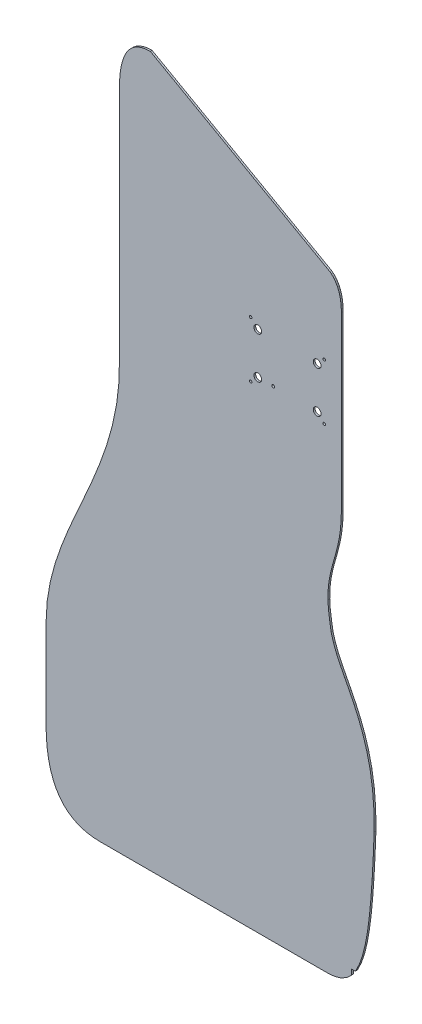
SolidWorks part; units mm, degrees
ref_plane "前视基准面" through (0, 0, 0) normal (0, 0, 1) x (1, 0, 0)
ref_plane "上视基准面" through (0, 0, 0) normal (0, 1, 0) x (1, 0, 0)
ref_plane "右视基准面" through (0, 0, 0) normal (1, 0, 0) x (0, 0, -1)
other "Configuration Table"
sketch "草图1" plane through (0, 0, 0) normal (0, 0, 1) x (1, 0, 0)
  line L0 (103, 235) -> (-24.8333, 235)
  line L1 (-24.8333, 235) -> (-152.6667, 235)
  line L2 (-152.6667, 235) -> (-280.5, 235)
  line L3 (-280.5, 235) -> (-293.0357, 235.6378)
  line L4 (-293.0357, 235.6378) -> (-304.6429, 237.551)
  line L5 (-304.6429, 237.551) -> (-315.3214, 240.7398)
  line L6 (-315.3214, 240.7398) -> (-325.0714, 245.2041)
  line L7 (-325.0714, 245.2041) -> (-333.8929, 250.9439)
  line L8 (-333.8929, 250.9439) -> (-341.7857, 257.9592)
  line L9 (-341.7857, 257.9592) -> (-348.75, 266.25)
  line L10 (-348.75, 266.25) -> (-354.7857, 275.8163)
  line L11 (-354.7857, 275.8163) -> (-359.8929, 286.6582)
  line L12 (-359.8929, 286.6582) -> (-364.0714, 298.7755)
  line L13 (-364.0714, 298.7755) -> (-367.3214, 312.1684)
  line L14 (-367.3214, 312.1684) -> (-369.6429, 326.8367)
  line L15 (-369.6429, 326.8367) -> (-371.0357, 342.7806)
  line L16 (-371.0357, 342.7806) -> (-371.5, 360)
  line L17 (-371.5, 360) -> (-371.5, 410)
  line L18 (-371.5, 410) -> (-371.5, 460)
  line L19 (-371.5, 460) -> (-371.5, 510)
  line L20 (-371.5, 510) -> (-369.6073, 541.7165)
  line L21 (-369.6073, 541.7165) -> (-364.3178, 572.7114)
  line L22 (-364.3178, 572.7114) -> (-356.2141, 603.1815)
  line L23 (-356.2141, 603.1815) -> (-345.879, 633.3236)
  line L24 (-345.879, 633.3236) -> (-333.8952, 663.3345)
  line L25 (-333.8952, 663.3345) -> (-320.8455, 693.4111)
  line L26 (-320.8455, 693.4111) -> (-307.3125, 723.75)
  line L27 (-307.3125, 723.75) -> (-293.879, 754.5481)
  line L28 (-293.879, 754.5481) -> (-281.1277, 786.0022)
  line L29 (-281.1277, 786.0022) -> (-269.6414, 818.309)
  line L30 (-269.6414, 818.309) -> (-260.0027, 851.6655)
  line L31 (-260.0027, 851.6655) -> (-252.7945, 886.2682)
  line L32 (-252.7945, 886.2682) -> (-248.5993, 922.3141)
  line L33 (-248.5993, 922.3141) -> (-248, 960)
  line L34 (-248, 960) -> (-248, 1090)
  line L35 (-248, 1090) -> (-248, 1220)
  line L36 (-248, 1220) -> (-248, 1350)
  line L37 (-248, 1350) -> (-247.7347, 1361.0204)
  line L38 (-247.7347, 1361.0204) -> (-246.9388, 1371.2245)
  line L39 (-246.9388, 1371.2245) -> (-245.6122, 1380.6122)
  line L40 (-245.6122, 1380.6122) -> (-243.7551, 1389.1837)
  line L41 (-243.7551, 1389.1837) -> (-241.3673, 1396.9388)
  line L42 (-241.3673, 1396.9388) -> (-238.449, 1403.8776)
  line L43 (-238.449, 1403.8776) -> (-235, 1410)
  line L44 (-235, 1410) -> (-231.0204, 1415.3061)
  line L45 (-231.0204, 1415.3061) -> (-226.5102, 1419.7959)
  line L46 (-226.5102, 1419.7959) -> (-221.4694, 1423.4694)
  line L47 (-221.4694, 1423.4694) -> (-215.898, 1426.3265)
  line L48 (-215.898, 1426.3265) -> (-209.7959, 1428.3673)
  line L49 (-209.7959, 1428.3673) -> (-203.1633, 1429.5918)
  line L50 (-203.1633, 1429.5918) -> (-196, 1430)
  line L51 (-196, 1430) -> (-95.25, 1373.3333)
  line L52 (-95.25, 1373.3333) -> (5.5, 1316.6667)
  line L53 (5.5, 1316.6667) -> (106.25, 1260)
  line L54 (106.25, 1260) -> (108.9362, 1257.8878)
  line L55 (108.9362, 1257.8878) -> (111.4235, 1255.551)
  line L56 (111.4235, 1255.551) -> (113.7117, 1252.9898)
  line L57 (113.7117, 1252.9898) -> (115.801, 1250.2041)
  line L58 (115.801, 1250.2041) -> (117.6913, 1247.1939)
  line L59 (117.6913, 1247.1939) -> (119.3827, 1243.9592)
  line L60 (119.3827, 1243.9592) -> (120.875, 1240.5)
  line L61 (120.875, 1240.5) -> (122.1684, 1236.8163)
  line L62 (122.1684, 1236.8163) -> (123.2628, 1232.9082)
  line L63 (123.2628, 1232.9082) -> (124.1582, 1228.7755)
  line L64 (124.1582, 1228.7755) -> (124.8546, 1224.4184)
  line L65 (124.8546, 1224.4184) -> (125.352, 1219.8367)
  line L66 (125.352, 1219.8367) -> (125.6505, 1215.0306)
  line L67 (125.6505, 1215.0306) -> (125.75, 1210)
  line L68 (125.75, 1210) -> (125.75, 1113.3333)
  line L69 (125.75, 1113.3333) -> (125.75, 1016.6667)
  line L70 (125.75, 1016.6667) -> (125.75, 920)
  line L71 (125.75, 920) -> (125.281, 904.7303)
  line L72 (125.281, 904.7303) -> (123.9876, 890.9038)
  line L73 (123.9876, 890.9038) -> (122.0405, 878.2799)
  line L74 (122.0405, 878.2799) -> (119.6101, 866.6181)
  line L75 (119.6101, 866.6181) -> (116.867, 855.6778)
  line L76 (116.867, 855.6778) -> (113.9818, 845.2187)
  line L77 (113.9818, 845.2187) -> (111.125, 835)
  line L78 (111.125, 835) -> (108.4672, 824.7813)
  line L79 (108.4672, 824.7813) -> (106.1789, 814.3222)
  line L80 (106.1789, 814.3222) -> (104.4308, 803.3819)
  line L81 (104.4308, 803.3819) -> (103.3932, 791.7201)
  line L82 (103.3932, 791.7201) -> (103.2369, 779.0962)
  line L83 (103.2369, 779.0962) -> (104.1323, 765.2697)
  line L84 (104.1323, 765.2697) -> (106.25, 750)
  line L85 (106.25, 750) -> (108.5868, 735.4045)
  line L86 (108.5868, 735.4045) -> (112.6079, 721.3994)
  line L87 (112.6079, 721.3994) -> (118.0076, 707.6567)
  line L88 (118.0076, 707.6567) -> (124.4803, 693.8484)
  line L89 (124.4803, 693.8484) -> (131.7206, 679.6465)
  line L90 (131.7206, 679.6465) -> (139.4227, 664.723)
  line L91 (139.4227, 664.723) -> (147.2812, 648.75)
  line L92 (147.2812, 648.75) -> (154.9905, 631.3994)
  line L93 (154.9905, 631.3994) -> (162.245, 612.3433)
  line L94 (162.245, 612.3433) -> (168.7391, 591.2536)
  line L95 (168.7391, 591.2536) -> (174.1672, 567.8025)
  line L96 (174.1672, 567.8025) -> (178.2238, 541.6618)
  line L97 (178.2238, 541.6618) -> (180.6032, 512.5036)
  line L98 (180.6032, 512.5036) -> (181, 480)
  line L99 (181, 480) -> (179.4934, 443.1706)
  line L100 (179.4934, 443.1706) -> (177.7026, 409.7522)
  line L101 (177.7026, 409.7522) -> (175.5423, 379.6356)
  line L102 (175.5423, 379.6356) -> (172.9271, 352.7114)
  line L103 (172.9271, 352.7114) -> (169.7719, 328.8703)
  line L104 (169.7719, 328.8703) -> (165.9913, 308.0029)
  line L105 (165.9913, 308.0029) -> (161.5, 290)
  line L106 (161.5, 290) -> (156.2128, 274.7522)
  line L107 (156.2128, 274.7522) -> (150.0445, 262.1501)
  line L108 (150.0445, 262.1501) -> (142.9096, 252.0845)
  line L109 (142.9096, 252.0845) -> (134.723, 244.4461)
  line L110 (134.723, 244.4461) -> (125.3994, 239.1254)
  line L111 (125.3994, 239.1254) -> (114.8535, 236.0131)
  line L112 (114.8535, 236.0131) -> (103, 235)
  point P0 (0, 0)
  dimension "D1" = 0.4643
  dimension "D2" = 1.8571
  dimension "D3" = 1.8927
  dimension "D4" = 4.1786
  dimension "D5" = 7.1822
  dimension "D6" = 7.4286
  dimension "D7" = 11.6071
  dimension "D8" = 15.2859
  dimension "D9" = 16.7143
  dimension "D10" = 22.75
  dimension "D11" = 25.621
  dimension "D12" = 29.7143
  dimension "D13" = 37.6048
  dimension "D14" = 37.6071
  dimension "D15" = 46.4286
  dimension "D16" = 50.6545
  dimension "D17" = 56.1786
  dimension "D18" = 64.1875
  dimension "D19" = 66.8571
  dimension "D20" = 77.621
  dimension "D21" = 78.4643
  dimension "D22" = 90.3723
  dimension "D23" = 91
  dimension "D24" = 101.8586
  dimension "D25" = 111.4973
  dimension "D26" = 118.7055
  dimension "D27" = 122.9007
  dimension "D28" = 123.5
  dimension "D29" = 123.7653
  dimension "D30" = 124.5612
  dimension "D31" = 125.8878
  dimension "D32" = 127.7449
  dimension "D33" = 130.1327
  dimension "D34" = 133.051
  dimension "D35" = 136.5
  dimension "D36" = 140.4796
  dimension "D37" = 144.9898
  dimension "D38" = 150.0306
  dimension "D39" = 155.602
  dimension "D40" = 161.7041
  dimension "D41" = 168.3367
  dimension "D42" = 175.5
  dimension "D43" = 218.8333
  dimension "D44" = 276.25
  dimension "D45" = 346.6667
  dimension "D46" = 371.5
  dimension "D47" = 377
  dimension "D48" = 474.5
  dimension "D49" = 474.7369
  dimension "D50" = 474.8932
  dimension "D51" = 475.6323
  dimension "D52" = 475.9308
  dimension "D53" = 477.6789
  dimension "D54" = 477.75
  dimension "D55" = 479.9672
  dimension "D56" = 480.0868
  dimension "D57" = 480.4362
  dimension "D58" = 482.625
  dimension "D59" = 482.9235
  dimension "D60" = 484.1079
  dimension "D61" = 485.2117
  dimension "D62" = 485.4818
  dimension "D63" = 486.3535
  dimension "D64" = 487.301
  dimension "D65" = 488.367
  dimension "D66" = 489.1913
  dimension "D67" = 489.5076
  dimension "D68" = 490.8827
  dimension "D69" = 491.1101
  dimension "D70" = 492.375
  dimension "D71" = 493.5405
  dimension "D72" = 493.6684
  dimension "D73" = 494.7628
  dimension "D74" = 495.4876
  dimension "D75" = 495.6582
  dimension "D76" = 495.9803
  dimension "D77" = 496.3546
  dimension "D78" = 496.781
  dimension "D79" = 496.852
  dimension "D80" = 496.8994
  dimension "D81" = 497.1505
  dimension "D82" = 497.25
  dimension "D83" = 503.2206
  dimension "D84" = 506.223
  dimension "D85" = 510.9227
  dimension "D86" = 514.4096
  dimension "D87" = 518.7812
  dimension "D88" = 521.5445
  dimension "D89" = 526.4905
  dimension "D90" = 527.7128
  dimension "D91" = 533
  dimension "D92" = 533.745
  dimension "D93" = 537.4913
  dimension "D94" = 540.2391
  dimension "D95" = 541.2719
  dimension "D96" = 544.4271
  dimension "D97" = 545.6672
  dimension "D98" = 547.0423
  dimension "D99" = 549.2026
  dimension "D100" = 549.7238
  dimension "D101" = 550.9934
  dimension "D102" = 552.1032
  dimension "D103" = 552.5
  dimension "D104" = 0.6378
  dimension "D105" = 1.0131
  dimension "D106" = 2.551
  dimension "D107" = 4.1254
  dimension "D108" = 5.7398
  dimension "D109" = 9.4461
  dimension "D110" = 10.2041
  dimension "D111" = 15.9439
  dimension "D112" = 17.0845
  dimension "D113" = 22.9592
  dimension "D114" = 27.1501
  dimension "D115" = 31.25
  dimension "D116" = 39.7522
  dimension "D117" = 40.8163
  dimension "D118" = 51.6582
  dimension "D119" = 55
  dimension "D120" = 63.7755
  dimension "D121" = 73.0029
  dimension "D122" = 77.1684
  dimension "D123" = 91.8367
  dimension "D124" = 93.8703
  dimension "D125" = 107.7806
  dimension "D126" = 117.7114
  dimension "D127" = 125
  dimension "D128" = 144.6356
  dimension "D129" = 174.7522
  dimension "D130" = 175
  dimension "D131" = 208.1706
  dimension "D132" = 225
  dimension "D133" = 245
  dimension "D134" = 275
  dimension "D135" = 277.5036
  dimension "D136" = 306.6618
  dimension "D137" = 306.7165
  dimension "D138" = 332.8025
  dimension "D139" = 337.7114
  dimension "D140" = 356.2536
  dimension "D141" = 368.1815
  dimension "D142" = 377.3433
  dimension "D143" = 396.3994
  dimension "D144" = 398.3236
  dimension "D145" = 413.75
  dimension "D146" = 428.3345
  dimension "D147" = 429.723
  dimension "D148" = 444.6465
  dimension "D149" = 458.4111
  dimension "D150" = 458.8484
  dimension "D151" = 472.6567
  dimension "D152" = 486.3994
  dimension "D153" = 488.75
  dimension "D154" = 500.4045
  dimension "D155" = 515
  dimension "D156" = 519.5481
  dimension "D157" = 530.2697
  dimension "D158" = 544.0962
  dimension "D159" = 551.0022
  dimension "D160" = 556.7201
  dimension "D161" = 568.3819
  dimension "D162" = 579.3222
  dimension "D163" = 583.309
  dimension "D164" = 589.7813
  dimension "D165" = 600
  dimension "D166" = 610.2187
  dimension "D167" = 616.6655
  dimension "D168" = 620.6778
  dimension "D169" = 631.6181
  dimension "D170" = 643.2799
  dimension "D171" = 651.2682
  dimension "D172" = 655.9038
  dimension "D173" = 669.7303
  dimension "D174" = 685
  dimension "D175" = 687.3141
  dimension "D176" = 725
  dimension "D177" = 781.6667
  dimension "D178" = 855
  dimension "D179" = 878.3333
  dimension "D180" = 975
  dimension "D181" = 980.0306
  dimension "D182" = 984.8367
  dimension "D183" = 985
  dimension "D184" = 989.4184
  dimension "D185" = 993.7755
  dimension "D186" = 997.9082
  dimension "D187" = 1001.8163
  dimension "D188" = 1005.5
  dimension "D189" = 1008.9592
  dimension "D190" = 1012.1939
  dimension "D191" = 1015.2041
  dimension "D192" = 1017.9898
  dimension "D193" = 1020.551
  dimension "D194" = 1022.8878
  dimension "D195" = 1025
  dimension "D196" = 1081.6667
  dimension "D197" = 1115
  dimension "D198" = 1126.0204
  dimension "D199" = 1136.2245
  dimension "D200" = 235
  dimension "D201" = 1145.6122
  dimension "D202" = 1154.1837
  dimension "D203" = 1161.9388
  dimension "D204" = 1168.8776
  dimension "D205" = 1175
  dimension "D206" = 1180.3061
  dimension "D207" = 1184.7959
  dimension "D208" = 1188.4694
  dimension "D209" = 1191.3265
  dimension "D210" = 1193.3673
  dimension "D211" = 1194.5918
extrude "凸台-拉伸1" add sketch "草图1" against normal mid plane 3
sketch "草图2" plane through (0, 0, 0) normal (0, 0, 1) x (1, 0, 0)
  line L0 (143, 239) -> (175, 239)
  line L1 (175, 239) -> (175, 261)
  line L2 (175, 261) -> (143, 261)
  line L3 (143, 261) -> (143, 239)
  line L4 (143, 1139) -> (175, 1139)
  line L5 (175, 1139) -> (175, 1161)
  line L6 (175, 1161) -> (143, 1161)
  line L7 (143, 1161) -> (143, 1139)
  point P0 (0, 0)
  dimension "D1" = 32
  dimension "D2" = 175
  dimension "D3" = 22
  dimension "D4" = 900
  dimension "D5" = 922
  dimension "D6" = 1161
extrude "切除-拉伸1" cut sketch "草图2" against normal mid plane 20
sketch "草图3" plane through (0, 0, 0) normal (0, 0, 1) x (1, 0, 0)
  circle A0 centre (-27, 1127) radius 2.25
  circle A1 centre (-27, 1033) radius 2.25
  circle A2 centre (97, 1127) radius 2.25
  circle A3 centre (97, 1033) radius 2.25
  circle A4 centre (-15, 1115) radius 6.5
  circle A5 centre (-15, 1045) radius 6.5
  circle A6 centre (85, 1115) radius 6.5
  circle A7 centre (85, 1045) radius 6.5
  circle A8 centre (11, 1045) radius 2.25
  point P0 (0, 0)
  dimension "D1" = 13
  dimension "D2" = 4.5
  dimension "D3" = 4.5
  dimension "D4" = 13
  dimension "D5" = 4.5
  dimension "D6" = 13
  dimension "D7" = 4.5
  dimension "D8" = 13
  dimension "D9" = 4.5
  dimension "D10" = 12
  dimension "D11" = 86
  dimension "D12" = 97
  dimension "D13" = 112
  dimension "D14" = 124
  dimension "D15" = 1033
  dimension "D16" = 1045
  dimension "D17" = 1115
  dimension "D18" = 1127
extrude "切除-拉伸2" cut sketch "草图3" against normal mid plane 10
